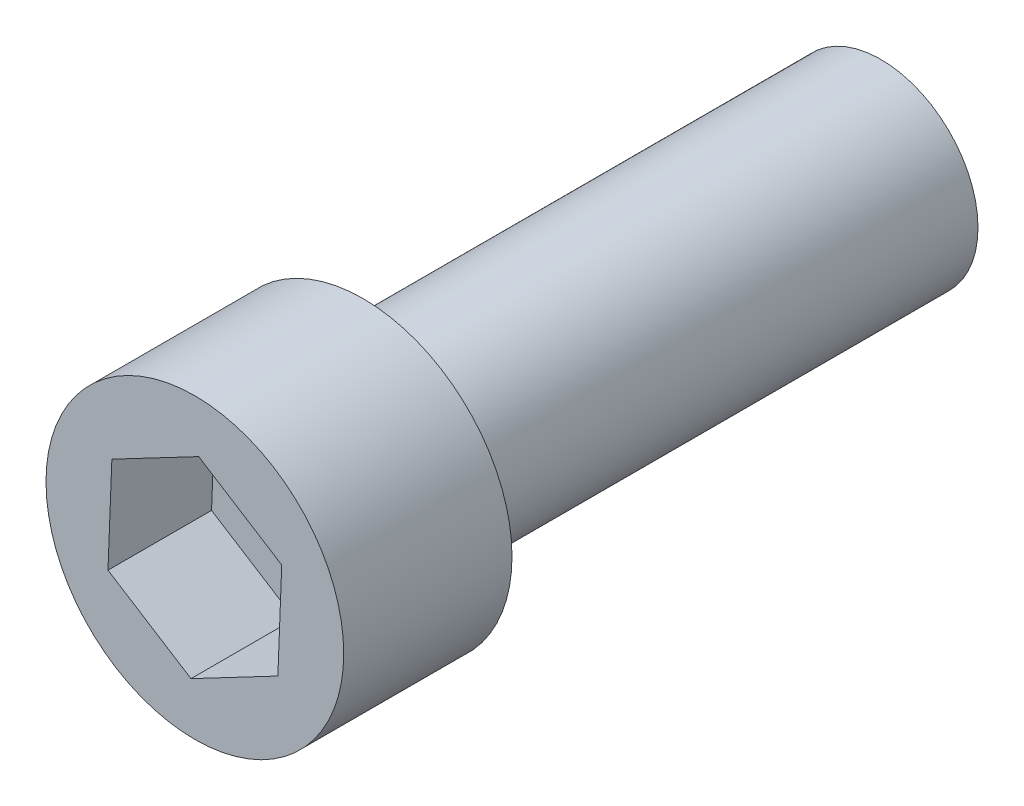
SolidWorks part; units mm, degrees
ref_plane "Front Plane" through (0, 0, 0) normal (0, 0, 1) x (1, 0, 0)
ref_plane "Top Plane" through (0, 0, 0) normal (0, 1, 0) x (1, 0, 0)
ref_plane "Right Plane" through (0, 0, 0) normal (1, 0, 0) x (0, 0, -1)
sketch "Sketch1" plane through (0, 0, 0) normal (0, 0, 1) x (1, 0, 0)
  circle A0 centre (0, 0) radius 7.5
  dimension "D1" = 15
extrude "Boss-Extrude1" add sketch "Sketch1" along normal blind 40
sketch "Sketch2" plane through (0, 0, 40) normal (0, 0, 1) x (1, 0, 0)
  circle A0 centre (0, 0) radius 11.5
  dimension "D1" = 23
extrude "Boss-Extrude2" add sketch "Sketch2" along normal blind 13
sketch "Sketch3" plane through (0, 0, 53) normal (0, 0, 1) x (1, 0, 0)
  line L1 (6.4121, -4.048) -> (6.7117, 3.5291)
  line L2 (6.7117, 3.5291) -> (0.2996, 7.5771)
  line L3 (0.2996, 7.5771) -> (-6.4121, 4.048)
  line L4 (-6.4121, 4.048) -> (-6.7117, -3.5291)
  line L5 (-6.7117, -3.5291) -> (-0.2996, -7.5771)
  line L6 (-0.2996, -7.5771) -> (6.4121, -4.048)
  circle A0 centre (0, 0) radius 6.5671 construction
extrude "Cut-Extrude1" cut sketch "Sketch3" against normal blind 8
